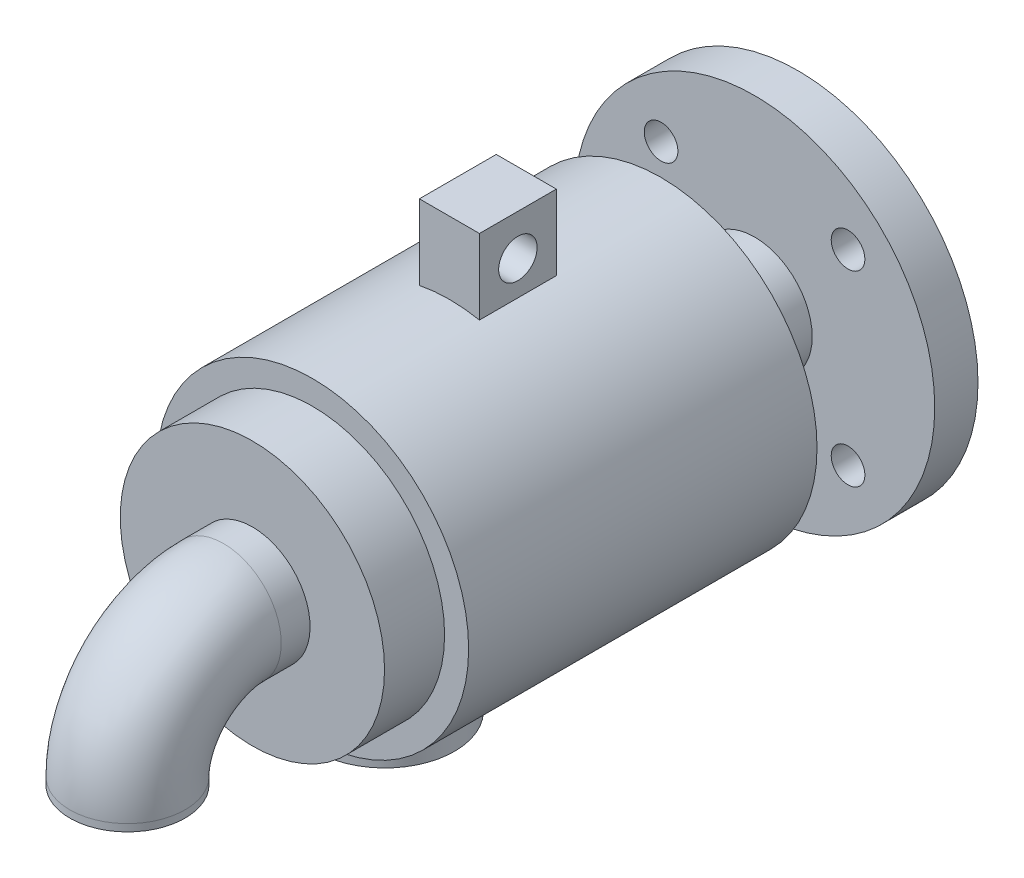
SolidWorks part; units mm, degrees
material "K"
ref_plane "Front" through (0, 0, 0) normal (0, 0, 1) x (1, 0, 0)
ref_plane "Top" through (0, 0, 0) normal (0, 1, 0) x (1, 0, 0)
ref_plane "Right" through (0, 0, 0) normal (1, 0, 0) x (0, 0, -1)
sketch "Sketch1" plane through (0, 0, 0) normal (0, 0, 1) x (1, 0, 0)
  circle A0 centre (0, 0) radius 75
  dimension "D1" = 150
extrude "Boss-Extrude1" add sketch "Sketch1" along normal blind 18
sketch "Sketch2" plane through (0, 0, 18) normal (0, 0, 1) x (1, 0, 0)
  circle A0 centre (0, 0) radius 24
  dimension "D1" = 48
extrude "Cut-Extrude1" cut sketch "Sketch2" against normal blind 12
sketch "Sketch3" plane through (0, 0, 0) normal (1, 0, 0) x (0, 0, -1)
  line L0 (12, 0) -> (-239, 0)
  line L1 (-279, -40) -> (-279, -43)
  line L2 (0, -75) -> (0, 75) construction
  arc A0 (-239, 0) -> (-279, -40) centre (-239, -40) ccw
  dimension "D3" = 40
  dimension "D1" = 12
  dimension "D2" = 291
  dimension "D4" = 43
ref_plane "Plane1" through (0, 0, -12) normal (0, 0, -1) x (-1, 0, 0)
sketch "Sketch5" plane through (0, 0, -12) normal (0, 0, -1) x (-1, 0, 0)
  circle A0 centre (0, 0) radius 24
sweep "Sweep1" add profiles "Sketch5" path "Sketch3"
ref_plane "Plane2" through (0, 0, 57) normal (0, 0, -1) x (-1, 0, 0)
sketch "Sketch6" plane through (0, 0, 57) normal (0, 0, -1) x (-1, 0, 0)
  circle A0 centre (0, 0) radius 65
  dimension "D1" = 130
extrude "Boss-Extrude2" add sketch "Sketch6" against normal blind 170
sketch "Sketch7" plane through (0, 0, 0) normal (0, 0, -1) x (-1, 0, 0)
  line L0 (0, 0) -> (-38.9059, 38.9059) construction
  line L1 (0, 0) -> (0, 60.6327) construction
  circle A0 centre (0, 0) radius 55 construction
  dimension "D2" = 110
  dimension "D1" = 45
hole_wizard "Ø14.0 (14) Hole1" positions "Sketch9" profile "Sketch8" hole size "Ø14.0" standard "GB"
sketch "Sketch9" plane through (0, 0, 0) normal (0, 0, -1) x (-1, 0, 0)
  point P0 (-38.9059, 38.9059)
sketch "Sketch8" plane through (38.9059, 38.9059, 0) normal (1, 0, 0) x (0, 1, 0)
  line L0 (0, 0) -> (0, 18)
  line L1 (0, 18) -> (7, 18)
  line L2 (7, 18) -> (7, 0)
  line L5 (7, 0) -> (0, 0)
  line L11 (0, -6.35) -> (0, 107.95) construction
  dimension "通孔孔直径" = 14
  dimension "通孔孔深度" = 18
pattern_circular "CirPattern1" count 4 over 360 about axis through (0, 0, 0) along (0, 0, 1) of "Ø14.0 (14) Hole1"
sketch "Sketch10" plane through (0, 0, 0) normal (0, 1, 0) x (1, 0, 0)
  circle A0 centre (0, -171.8439) radius 29
  dimension "D1" = 58
extrude "Boss-Extrude3" add sketch "Sketch10" against normal blind 70
sketch "Sketch11" plane through (0, 0, -12) normal (0, 0, -1) x (-1, 0, 0)
  circle A0 centre (0, 0) radius 19
  dimension "D1" = 38
extrude "Cut-Extrude2" cut sketch "Sketch11" against normal blind 187
sketch "Sketch12" plane through (0, 0, 0) normal (1, 0, 0) x (0, 0, -1)
  line L0 (-279, -43) -> (-279, -30)
  line L1 (-303, -43) -> (-255, -43) construction
  line L2 (-249, 0) -> (-239, 0)
  line L3 (-239, 24) -> (-239, -24) construction
  arc A0 (-249, 0) -> (-279, -30) centre (-249, -30) ccw
  dimension "D1" = 30
sketch "Sketch13" plane through (0, -43, 0) normal (0, -1, 0) x (1, 0, 0)
  circle A0 centre (0, 279) radius 12.5
  dimension "D1" = 25
sweep "Cut-Sweep1" cut profiles "Sketch13" path "Sketch12"
cosmetic thread "Cosmetic Thread2" parameters "D2"=32.8422
sketch "Sketch14" plane through (0, 0, 227) normal (0, 0, 1) x (1, 0, 0)
  circle A0 centre (0, 0) radius 65
  circle A1 centre (0, 0) radius 55
  dimension "D1" = 110
extrude "Cut-Extrude3" cut sketch "Sketch14" against normal blind 25
sketch "Sketch15" plane through (0, -70, 0) normal (0, -1, 0) x (-1, 0, 0)
  circle A0 centre (0, -171.8439) radius 24
  dimension "D1" = 48
extrude "Cut-Extrude4" cut sketch "Sketch15" against normal blind 60
cosmetic thread "Cosmetic Thread1" parameters "D2"=59.7154
sketch "Sketch16" plane through (0, 0, 0) normal (1, 0, 0) x (0, 0, -1)
  line L0 (12, -24) -> (12, 24) construction
  line L1 (-145, 23.9369) -> (-113, 23.9369)
  line L2 (-145, 23.9369) -> (-145, 95)
  line L3 (-145, 95) -> (-113, 95)
  line L4 (-113, 23.9369) -> (-113, 95)
  line L6 (0, 0) -> (-181.0414, 0) construction
  dimension "D1" = 32
  dimension "D2" = 125
  dimension "D3" = 95
extrude "Boss-Extrude4" add sketch "Sketch16" along normal mid plane 25
sketch "Sketch17" plane through (12.5, 0, 0) normal (1, 0, 0) x (0, 0, -1)
  line L0 (-129, 95) -> (-129, 61) construction
  line L1 (-113, 95) -> (-145, 95) construction
  line L2 (-57, 0) -> (-145.7056, 0) construction
  line L3 (-57, -65) -> (-57, 65) construction
  circle A0 centre (-129, 78) radius 8
  dimension "D1" = 78
  dimension "D2" = 16
extrude "Cut-Extrude5" cut sketch "Sketch17" against normal blind 25
equation "\"零件重量\"= IIF ( \"SW-质量\" > 100 , int ( \"SW-质量\" ) , \"SW-质量\" )"
